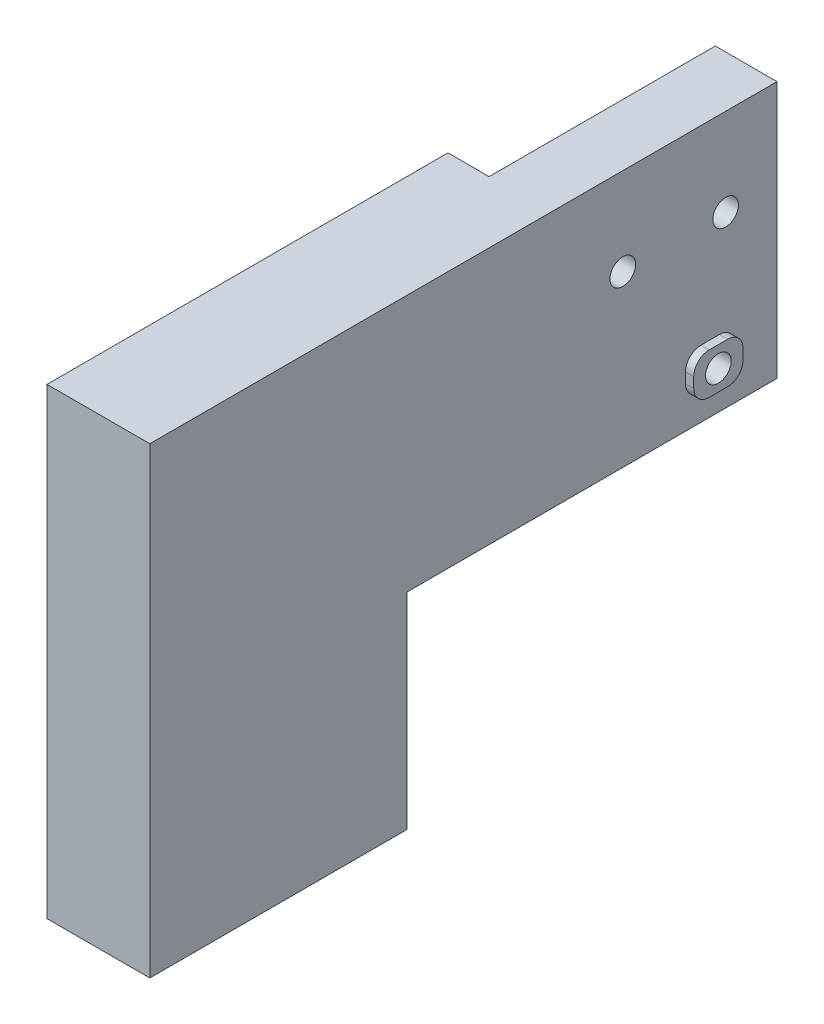
from build123d import *

# Parameters (mm, degrees)
EXTRUDE_THIN1_DEPTH   = 25
SKETCH2_W             = 36
SKETCH2_H             = 25
BOSS_EXTRUDE1_DEPTH   = 10
SKETCH5_W             = 4
SKETCH5_H             = 22
CUT_EXTRUDE1_DEPTH    = 68.424031324
SKETCH6_W             = 93.972678959
SKETCH6_H             = 54.427614962
CUT_EXTRUDE2_DEPTH    = 10
M5_TAPPED_HOLE1_D     = 4.2
M5_TAPPED_HOLE1_DEPTH = 12.4
M5_TAPPED_HOLE1_TIP   = 1.2618073
M3_TAPPED_HOLE1_D     = 2.5
SKETCH12_W            = 4.8
SKETCH12_H            = 4
BOSS_EXTRUDE2_DEPTH   = 0.8
M3_TAPPED_HOLE2_D     = 2.5
FILLET1_R             = 1.5


with BuildPart() as part:
    # Sketch1 → Extrude-Thin1 (new body)
    with BuildSketch(Plane.XY):
        Polygon((-15, 0), (0, 0), (0, 45), (10, 45), (10, -10), (-15, -10), align=None)
    extrude(amount=EXTRUDE_THIN1_DEPTH)

    # Sketch2 → Boss-Extrude1 (add)
    with BuildSketch(Plane.ZY):
        with Locations((-18, 32.5)):
            Rectangle(SKETCH2_W, SKETCH2_H)
    extrude(amount=-BOSS_EXTRUDE1_DEPTH)

    # Sketch5 → Cut-Extrude1 (cut, through all)
    with BuildSketch(Plane(origin=(0, 45, 0), x_dir=(1, 0, 0), z_dir=(0, 1, 0))):
        with Locations((2, 25)):
            Rectangle(SKETCH5_W, SKETCH5_H)
    extrude(amount=-CUT_EXTRUDE1_DEPTH, mode=Mode.SUBTRACT)

    # Sketch6 → Cut-Extrude2 (cut)
    with BuildSketch(Plane.XZ.offset(10)):
        with Locations((-13.059524258, 16.160355611)):
            Rectangle(SKETCH6_W, SKETCH6_H)
    extrude(amount=-CUT_EXTRUDE2_DEPTH, mode=Mode.SUBTRACT)

    # M5 Tapped Hole1
    with Locations(Plane(origin=(0, 0, 0), x_dir=(-1, 0, 0), z_dir=(0, -1, 0))):
        with Locations((-5, -5.5), (-5, -19.5)):
            Hole(M5_TAPPED_HOLE1_D / 2, depth=M5_TAPPED_HOLE1_DEPTH)
            with Locations((0, 0, -(M5_TAPPED_HOLE1_DEPTH + M5_TAPPED_HOLE1_TIP / 2))):  # 118° drill point
                Cone(0, M5_TAPPED_HOLE1_D / 2, M5_TAPPED_HOLE1_TIP, mode=Mode.SUBTRACT)

    # M3 Tapped Hole1 (through all)
    with Locations(Plane(origin=(10, 0, 0), x_dir=(0, 0, -1), z_dir=(1, 0, 0))):
        with Locations((21, 36.5), (31, 36.5)):
            Hole(M3_TAPPED_HOLE1_D / 2)

    # Sketch12 → Boss-Extrude2 (add)
    with BuildSketch(Plane(origin=(10, 0, 0), x_dir=(0, 0, -1), z_dir=(1, 0, 0))):
        with Locations((29.5, 24.5)):
            Rectangle(SKETCH12_W, SKETCH12_H)
    extrude(amount=BOSS_EXTRUDE2_DEPTH)

    # M3 Tapped Hole2 (through all)
    with Locations(Plane.ZY):
        with Locations((-29.5, 24.5)):
            Hole(M3_TAPPED_HOLE2_D / 2)

    # Fillet1
    fillet1_edges = [part.edges().sort_by_distance(p)[0] for p in [
        (10.4, 22.5, -31.9),
        (10.4, 26.5, -31.9),
        (10.4, 26.5, -27.1),
        (10.4, 22.5, -27.1),
    ]]
    fillet(fillet1_edges, radius=FILLET1_R)


solid = part.part
